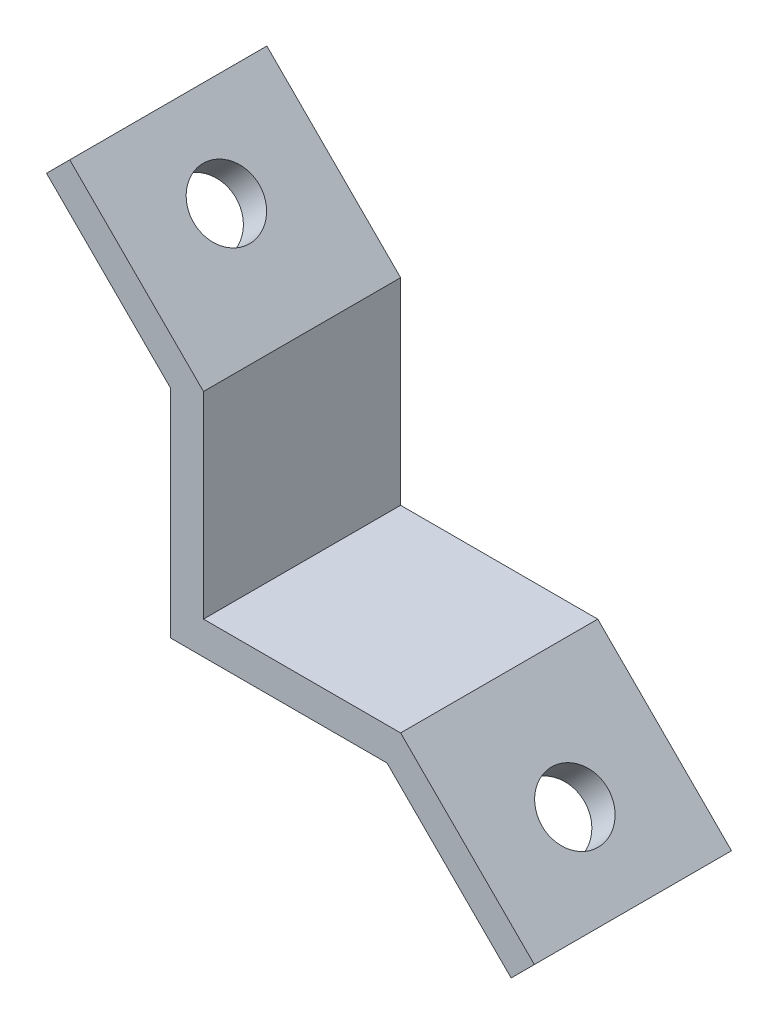
from build123d import *

# Parameters (mm, degrees)
EXTRUDE_1_DEPTH     = 60
EXTRUDE_2_DEPTH     = 60
SKETCH_3_R          = 10
CUT_EXTRUDE_1_DEPTH = 60


with BuildPart() as part:
    # 草图1 → 凸台-拉伸1 (new body)
    with BuildSketch(Plane.XY):
        Polygon((0, 0), (0, 60), (-10, 60), (-10, -10), (60, -10), (60, 0), align=None)
    extrude(amount=EXTRUDE_1_DEPTH)

    # 草图2 → 凸台-拉伸2 (add)
    with BuildSketch(Plane.XY):
        Polygon((0, 60), (-40.710678119, 100.710678119), (-47.781745931, 93.639610307), (-10, 55.857864376), (-10, 60), align=None)
        Polygon((60, 0), (100.710678119, -40.710678119), (93.639610307, -47.781745931), (55.857864376, -10), (60, -10), align=None)
    extrude(amount=EXTRUDE_2_DEPTH)

    # 草图3 → 切除-拉伸1 (cut)
    with BuildSketch(Plane(origin=(22.928932188, 22.928932188, 0), x_dir=(0, 0, 1), z_dir=(-0.7071067811865501, -0.7071067811865449, 0))):
        with Locations(Location((30, 75, 0), (0, 0, 270))):
            Circle(SKETCH_3_R)
        with Locations(Location((30, -75, 0), (0, 0, 270))):
            Circle(SKETCH_3_R)
    extrude(amount=-CUT_EXTRUDE_1_DEPTH, mode=Mode.SUBTRACT)


solid = part.part
